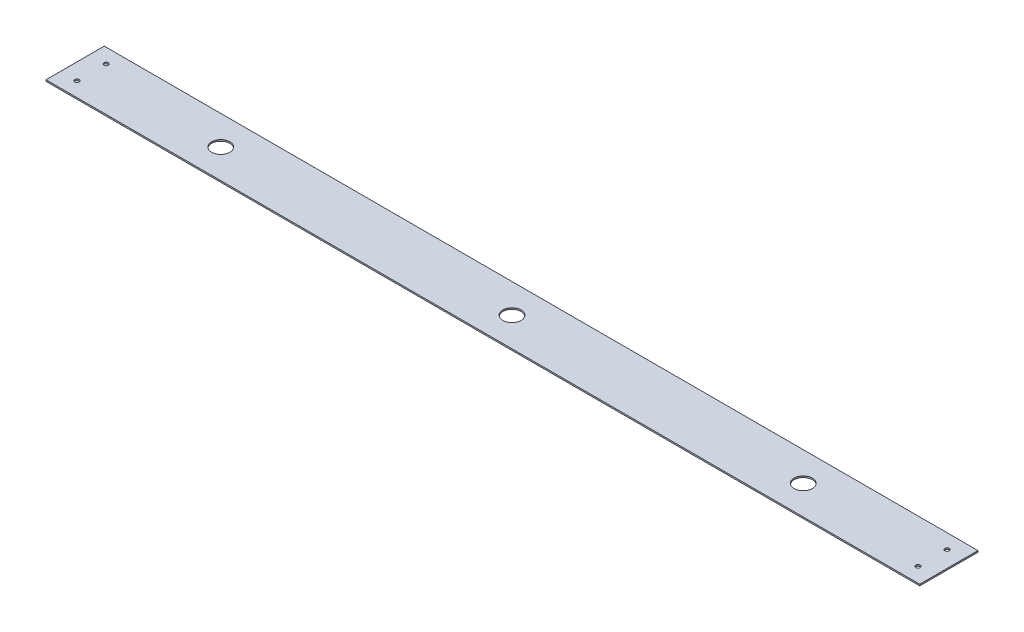
SolidWorks part; units mm, degrees
material "6061-T6 (GB)"
ref_plane "Front Plane" through (0, 0, 0) normal (0, 0, 1) x (1, 0, 0)
ref_plane "Top Plane" through (0, 0, 0) normal (0, 1, 0) x (1, 0, 0)
ref_plane "Right Plane" through (0, 0, 0) normal (1, 0, 0) x (0, 0, -1)
sketch "Sketch1" plane through (0, 0, 0) normal (0, 1, 0) x (1, 0, 0)
  line L0 (0, 40) -> (0, -40) construction
  line L1 (600, -40) -> (-600, -40)
  line L2 (600, -40) -> (600, 40)
  line L3 (600, 40) -> (-600, 40)
  line L4 (-600, -40) -> (-600, 40)
  line L5 (600, -40) -> (-600, 40) construction
  line L6 (600, 40) -> (-600, -40) construction
  line L7 (-600, 0) -> (600, 0) construction
  circle A0 centre (-400, 0) radius 12.5
  circle A1 centre (400, 0) radius 12.5
  circle A2 centre (-577.5, 20) radius 3
  circle A3 centre (577.5, 20) radius 3
  circle A4 centre (-577.5, -20) radius 3
  circle A5 centre (577.5, -20) radius 3
  circle A6 centre (0, 0) radius 12.5
  point P0 (0, 0)
  dimension "D3" = 800
  dimension "D4" = 25
  dimension "D6" = 22.5
  dimension "D7" = 6
  dimension "D8" = 40
  dimension "D1" = 80
  dimension "D2" = 1200
  dimension "D5" = 40
extrude "Boss-Extrude1" add sketch "Sketch1" along normal blind 2
